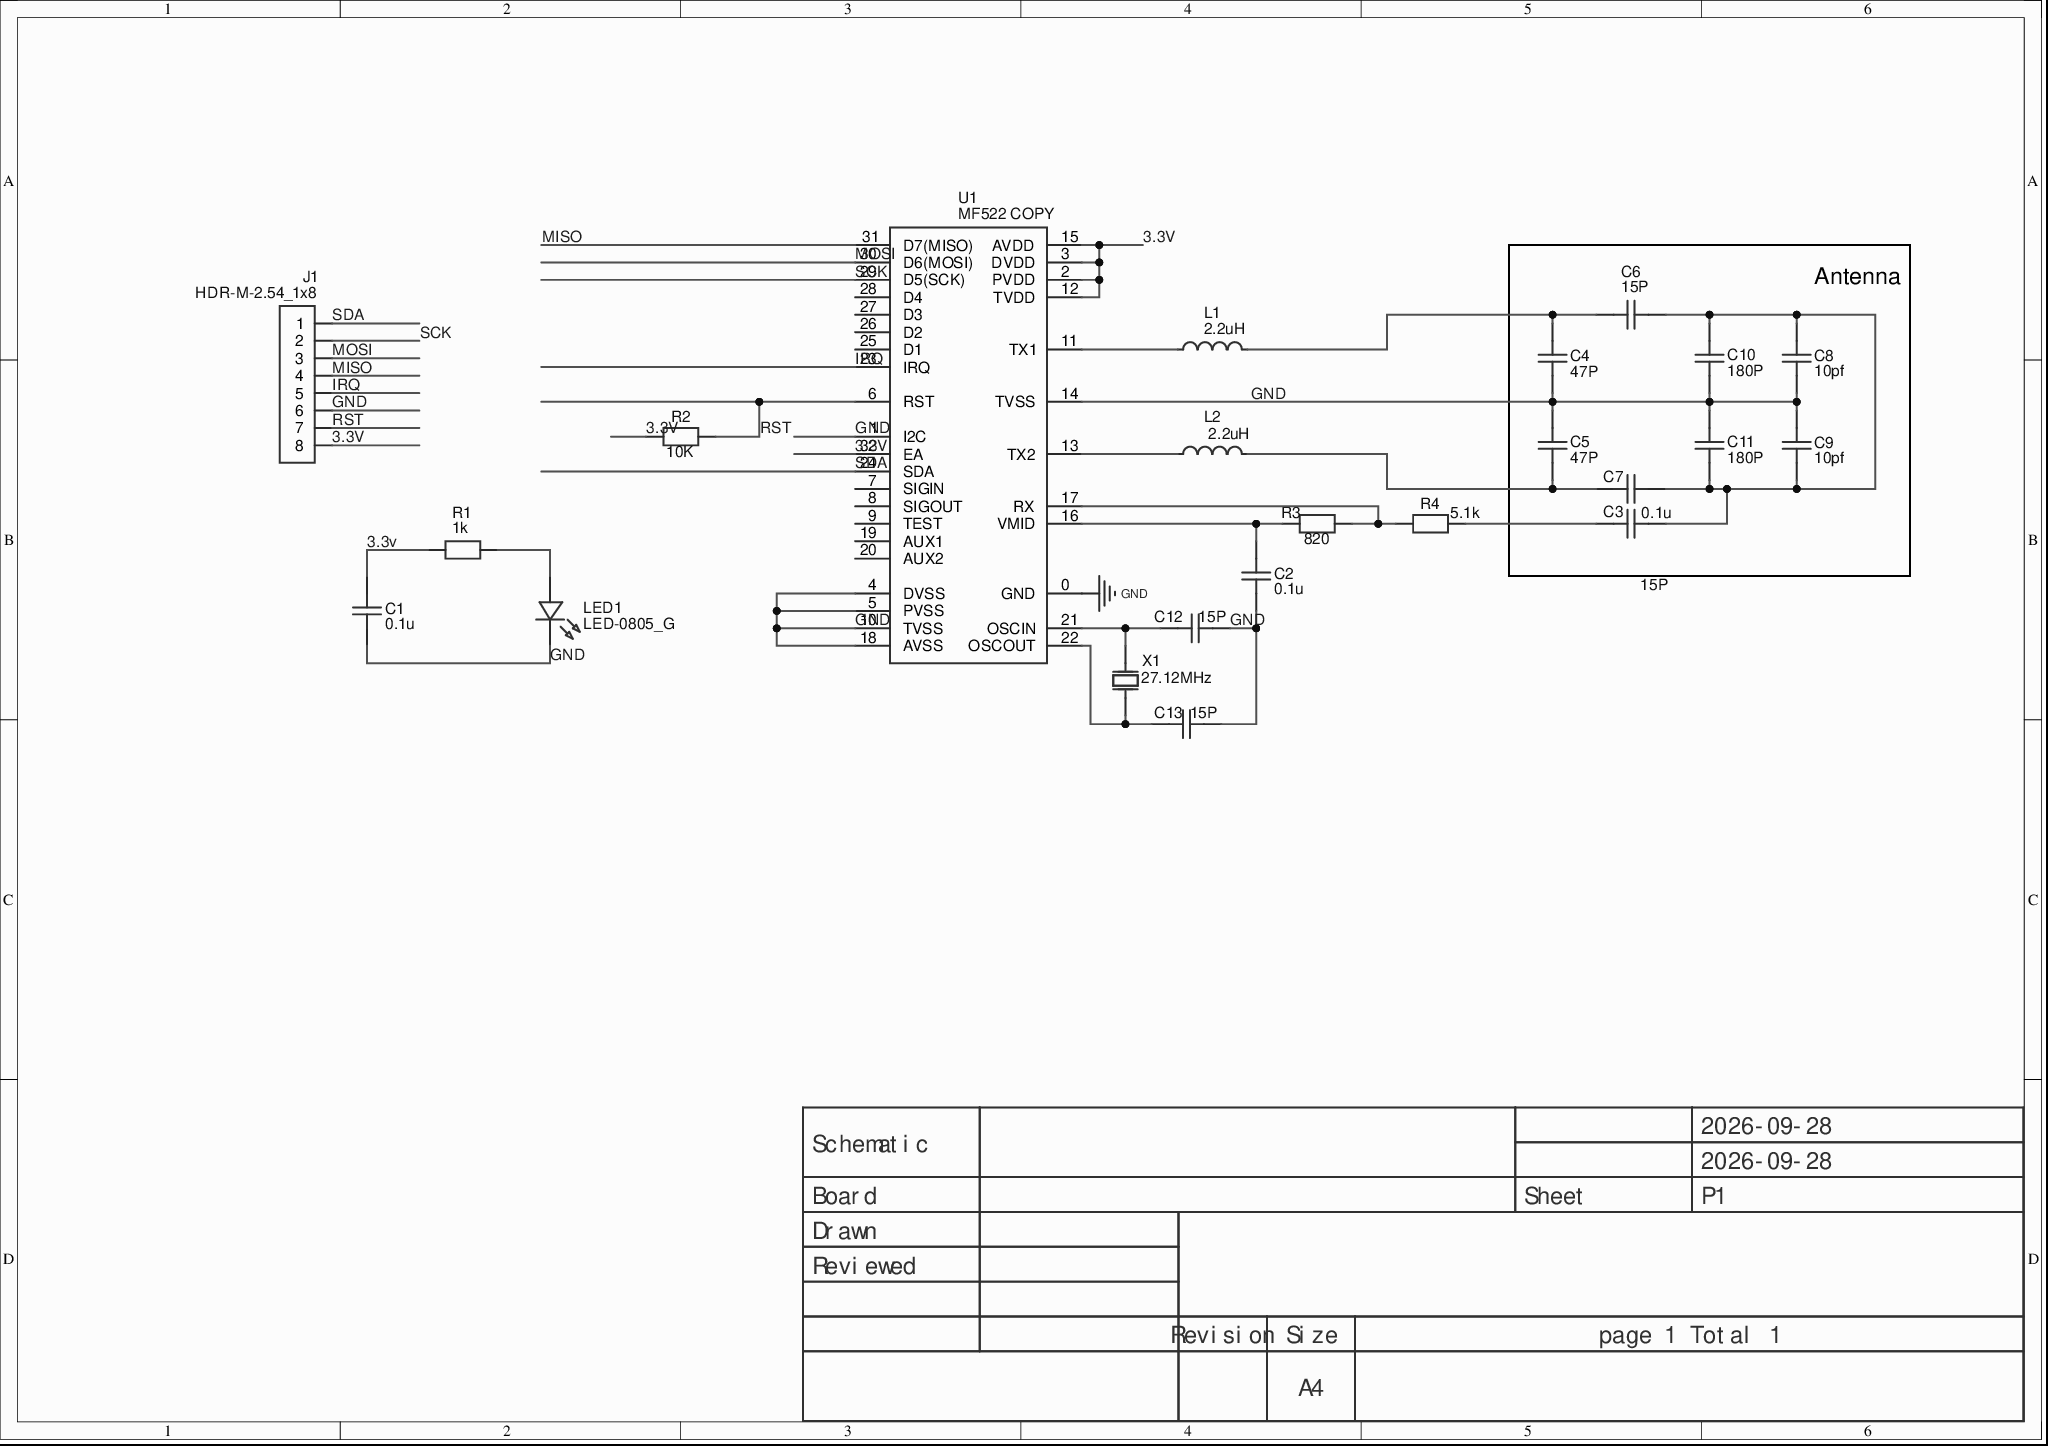
[diagram p0: MISC61972-3.schdoc]
# Altium project MISC61972-2.PrjPcb
1 sheet, 23 parts. Net scope: global (net labels, ports and power ports of the same name join across sheets).
Board file: MISC61972.pcbdoc

## Sheet MISC61972-3.schdoc
size 297 x 209 mm; Version: V1.0; @Project Name: MISC61972; @Update Date: 2026-09-28; @Create Date: 2026-09-28; @Board Name: MISC61972; @Create Time: 16:30:53; @Page Count: 1; @Page No: 1; @Schematic Name: MISC61972; @Update Time: 16:30:53; Size: A4

### Parts
C1  0.1u  [C0805]
C2  0.1u  [C0805]
C3  0.1u  [C0805]
C4  47P  [C0805]
C5  47P  [C0805]
C6  15P  [C0805]
C7  15P  [C0805]
C8  10pf  [C0805]
C9  10pf  [C0805]
C10  180P  [C0805]
C11  180P  [C0805]
C12  15P  [C0805]
C13  15P  [C0805]
J1  HDR-M-2.54_1x8  [HDR-M-2.54_1X8]
L1  2.2uH  [L0805]
L2  2.2uH  [L0805]
LED1  LED-0805_G  [LED-0805_G]
R1  1k  [R0805]
R2  10K  [R0805]
R3  820  [R0805]
R4  5.1k  [R0805]
U1  MF522 COPY  [LC-QFN-32_5X5X05P]
X1  27.12MHz  [HC-49US_L11.5-W4.5-P4.88]

### Blocks framed on the sheet
Antenna: C3-C11

### Nets
GND: C1.1 C2.1 C4.1 C5.2 C8.1 C9.2 C10.1 C11.2 C12.2 C13.2 J1.6 LED1.2 U1.0(GND) U1.1(I2C) U1.4(DVSS) U1.5(PVSS) U1.10(TVSS) U1.14(TVSS) U1.18(AVSS)
3.3V: C1.2 J1.8 R1.1 R2.1 U1.2(PVDD) U1.3(DVDD) U1.12(TVDD) U1.15(AVDD) U1.32(EA)
IRQ: J1.5 U1.23(IRQ)
MISO: J1.4 U1.31(D7(MISO))
MOSI: J1.3 U1.30(D6(MOSI))
RST: J1.7 R2.2 U1.6(RST)
SCK: J1.2 U1.29(D5(SCK))
SDA: J1.1 U1.24(SDA)
NetC2_2: C2.2 R3.1 U1.16(VMID)
NetC3_1: C3.1 R4.2
NetC3_2: C3.2 C6.2 C7.2 C8.2 C9.1 C10.2 C11.1
NetC4_2: C4.2 C6.1 L1.2
NetC5_1: C5.1 C7.1 L2.2
NetC12_1: C12.1 U1.21(OSCIN) X1.1(OSC1)
NetC13_1: C13.1 U1.22(OSCOUT) X1.2(OSC2)
NetL1_1: L1.1 U1.11(TX1)
NetL2_1: L2.1 U1.13(TX2)
NetLED1_1: LED1.1 R1.2
NetR3_2: R3.2 R4.1 U1.17(RX)

Not connected (* = marked no-connect by the designer): U1 7(SIGIN) 8(SIGOUT) 9(TEST) 19(AUX1) 20(AUX2) 25(D1) 26(D2) 27(D3) 28(D4)

### Notes on the sheet
- 2026-09-28
- Schematic
- Board
- Sheet
- P1
- Drawn
- Reviewed
- Revision
- Size
- A4
- page 1 Total 1

### Library data of the parts
C1-C3 = 0.1u: Add into BOM: yes; Symbol: 0.1u; Device: 0.1u; Convert to PCB: yes; Origin Footprint: C0805; FootprintName: C0805
C4 C5 = 47P: Add into BOM: yes; Symbol: 47P; Device: 47P; Convert to PCB: yes; Origin Footprint: C0805; FootprintName: C0805
C6 C7 C12 C13 = 15P: Add into BOM: yes; Symbol: 15P; Device: 15P; Convert to PCB: yes; Origin Footprint: C0805; FootprintName: C0805
C8 C9 = 10pf: Add into BOM: yes; Symbol: 10pf; Device: 10pf; Convert to PCB: yes; Origin Footprint: C0805; FootprintName: C0805
C10 C11 = 180P: Add into BOM: yes; Symbol: 180P; Device: 180P; Convert to PCB: yes; Origin Footprint: C0805; FootprintName: C0805
J1 = HDR-M-2.54_1x8: Add into BOM: yes; 3D Model: bc4c7d1499344595a34d06f657b047c00819f05c4eef4c71ace90d822a990e87; Symbol: HDR-M-2.54_1x8; Device: HDR-M-2.54_1x8; Convert to PCB: yes; Supplier Part: C190820; Supplier: LCSC; Origin Footprint: HDR-M-2.54_1X8; ModelName: HDR-M-2.54_1x8
L1 L2 = 2.2uH: Add into BOM: yes; Symbol: 2.2uH; Device: 2.2uH; Convert to PCB: yes; Origin Footprint: L0805; FootprintName: L0805
LED1 = NCD0805G1: Manufacturer: 国星光电; Add into BOM: yes; Origin Footprint: LED0805_GREEN; 3D Model: 1551dc45878a49c78968815de7a37f0b0819f05c4eef4c71ace90d822a990e87; Symbol: LED-0805_G; Device: NCD0805G1; Convert to PCB: yes; Manufacturer Part: NCD0805G1; Supplier Part: C84260; ModelName: LED0805_Green
R1 = 1k: Add into BOM: yes; 3D Model: 1f8f9bfd8e2b427398b06535d781678a0819f05c4eef4c71ace90d822a990e87; Symbol: 1k; Device: 1k; Convert to PCB: yes; Origin Footprint: R0805; FootprintName: R0805; ModelName: R0805
R2 = 10K: Add into BOM: yes; 3D Model: 1f8f9bfd8e2b427398b06535d781678a0819f05c4eef4c71ace90d822a990e87; Symbol: 10K; Device: 10K; Convert to PCB: yes; Origin Footprint: R0805; FootprintName: R0805; ModelName: R0805
R3 = 820: Add into BOM: yes; 3D Model: 1f8f9bfd8e2b427398b06535d781678a0819f05c4eef4c71ace90d822a990e87; Symbol: 820; Device: 820; Convert to PCB: yes; Origin Footprint: R0805; FootprintName: R0805; ModelName: R0805
R4 = 5.1k: Add into BOM: yes; 3D Model: 1f8f9bfd8e2b427398b06535d781678a0819f05c4eef4c71ace90d822a990e87; Symbol: 5.1k; Device: 5.1k; Convert to PCB: yes; Origin Footprint: R0805; FootprintName: R0805; ModelName: R0805
U1 = MF522 COPY: Add into BOM: yes; Symbol: MF522 COPY; Device: MF522 COPY; Convert to PCB: yes; Origin Footprint: LC-QFN-32_5X5X05P
X1 = X49UD196608MSD2SC: Manufacturer: null; Add into BOM: yes; Symbol: 27.12MHz; Device: X49UD196608MSD2SC; Convert to PCB: yes; Supplier: LCSC; Manufacturer Part: X49UD196608MSD2SC; Supplier Part: C2193; JLCPCB Part Class: Extended Part; Origin Footprint: HC-49US_L11.5-W4.5-P4.88